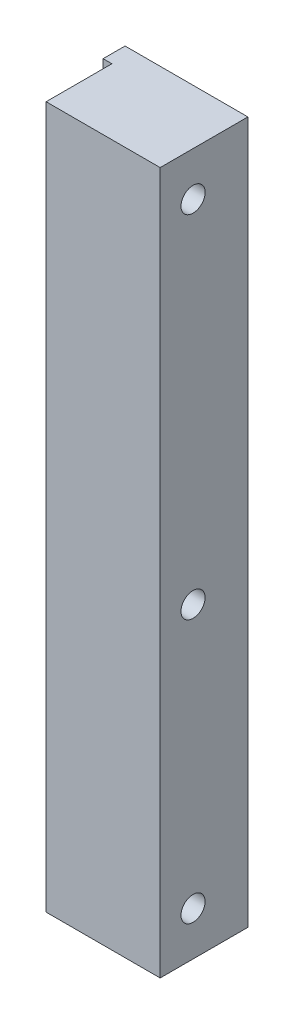
from build123d import *

# Parameters (mm, degrees)
SKETCH_1_W                                         = 20
SKETCH_1_H                                         = 160
BOSS_EXTRUDE_1_DEPTH                               = 28
SKETCH_2_W                                         = 15
SKETCH_2_H                                         = 160
CUT_EXTRUDE_1_DEPTH                                = 2
LINEAR_PATTERN_1_COUNT                             = 3
LINEAR_PATTERN_1_PITCH                             = 60
M5_SOCKET_HEAD_CAP_SCREW_COUNTERBORE_1_D           = 5.5
M5_SOCKET_HEAD_CAP_SCREW_COUNTERBORE_1_CBORE_D     = 10
M5_SOCKET_HEAD_CAP_SCREW_COUNTERBORE_1_CBORE_DEPTH = 5
LINEAR_PATTERN_2_COUNT                             = 2
LINEAR_PATTERN_2_PITCH                             = 140
LINEAR_PATTERN_3_COUNT                             = 2
LINEAR_PATTERN_3_PITCH                             = 60


with BuildPart() as part:
    # Sketch 1 → Boss-Extrude 1 (new body)
    with BuildSketch(Plane(origin=(0, 0, 0), x_dir=(0, 0, -1), z_dir=(1, 0, 0))):
        Rectangle(SKETCH_1_W, SKETCH_1_H)
    extrude(amount=BOSS_EXTRUDE_1_DEPTH)

    # Sketch 2 → Cut-Extrude 1 (cut)
    with BuildSketch(Plane.ZY):
        with Locations((2.5, 0)):
            Rectangle(SKETCH_2_W, SKETCH_2_H)
    extrude(amount=-CUT_EXTRUDE_1_DEPTH, mode=Mode.SUBTRACT)

    # Sketch 3 → M3 Tapped Hole 1 (revolve, cut)
    with BuildSketch(Plane(origin=(2, -60, 2.5), x_dir=(0, 0, 1), z_dir=(0, 1, 0))):
        Polygon((0, 0), (0, 8.251075774), (1.25, 7.5), (1.25, 0), align=None)
    m3_tapped_hole_1 = revolve(axis=Axis((-4.35, -60, 2.5), (1, 0, 0)), mode=Mode.SUBTRACT)

    # Linear Pattern 1: M3 Tapped Hole 1 ×3
    with Locations(*[(0, i * LINEAR_PATTERN_1_PITCH, 0) for i in range(1, LINEAR_PATTERN_1_COUNT)]):
        add(m3_tapped_hole_1, mode=Mode.SUBTRACT)

    # M5 Socket Head Cap Screw Counterbore 1 (through all)
    with Locations(Plane.ZY.offset(-2)):
        with Locations((2.5, -70)):
            m5_socket_head_cap_screw_counterbore_1 = CounterBoreHole(M5_SOCKET_HEAD_CAP_SCREW_COUNTERBORE_1_D / 2, M5_SOCKET_HEAD_CAP_SCREW_COUNTERBORE_1_CBORE_D / 2, M5_SOCKET_HEAD_CAP_SCREW_COUNTERBORE_1_CBORE_DEPTH)

    # Linear Pattern 2: M5 Socket Head Cap Screw Counterbore 1 ×2
    with Locations(*[(0, i * LINEAR_PATTERN_2_PITCH, 0) for i in range(1, LINEAR_PATTERN_2_COUNT)]):
        add(m5_socket_head_cap_screw_counterbore_1, mode=Mode.SUBTRACT)

    # Linear Pattern 3: M5 Socket Head Cap Screw Counterbore 1 ×2
    with Locations(*[(0, i * LINEAR_PATTERN_3_PITCH, 0) for i in range(1, LINEAR_PATTERN_3_COUNT)]):
        add(m5_socket_head_cap_screw_counterbore_1, mode=Mode.SUBTRACT)


solid = part.part
